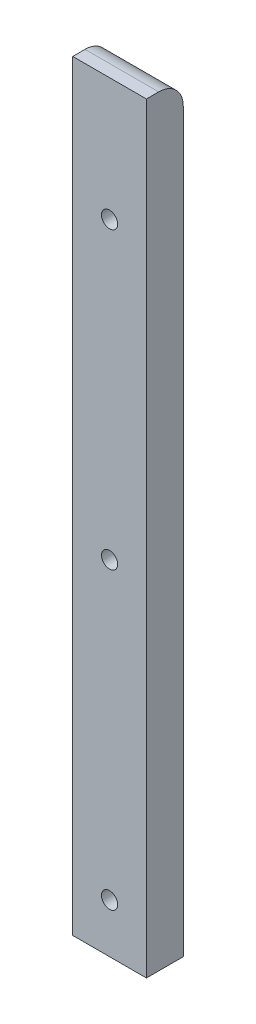
from build123d import *

# Parameters (mm, degrees)
SKETCH_1_W                = 30
SKETCH_1_H                = 310
EXTRUDE_1_DEPTH           = 15
HOLE_WIZARD_1_D           = 6.6
HOLE_WIZARD_1_CBORE_D     = 11
HOLE_WIZARD_1_CBORE_DEPTH = 6.8
FILLET_1_R                = 10


with BuildPart() as part:
    # 草图1 → 凸台-拉伸1 (new body)
    with BuildSketch(Plane.XY):
        Rectangle(SKETCH_1_W, SKETCH_1_H)
    extrude(amount=EXTRUDE_1_DEPTH)

    # 打孔尺寸(%根据)内六角圆柱头螺钉的类型1 (through all)
    with Locations(Plane(origin=(0, 0, 0), x_dir=(-1, 0, 0), z_dir=(0, 0, -1))):
        with Locations((0, 105), (0, -15), (0, -135)):
            CounterBoreHole(HOLE_WIZARD_1_D / 2, HOLE_WIZARD_1_CBORE_D / 2, HOLE_WIZARD_1_CBORE_DEPTH)

    # 圆角1
    fillet_1_edges = [part.edges().sort_by_distance(p)[0] for p in [
        (0, 155, 0),
    ]]
    fillet(fillet_1_edges, radius=FILLET_1_R)


solid = part.part
